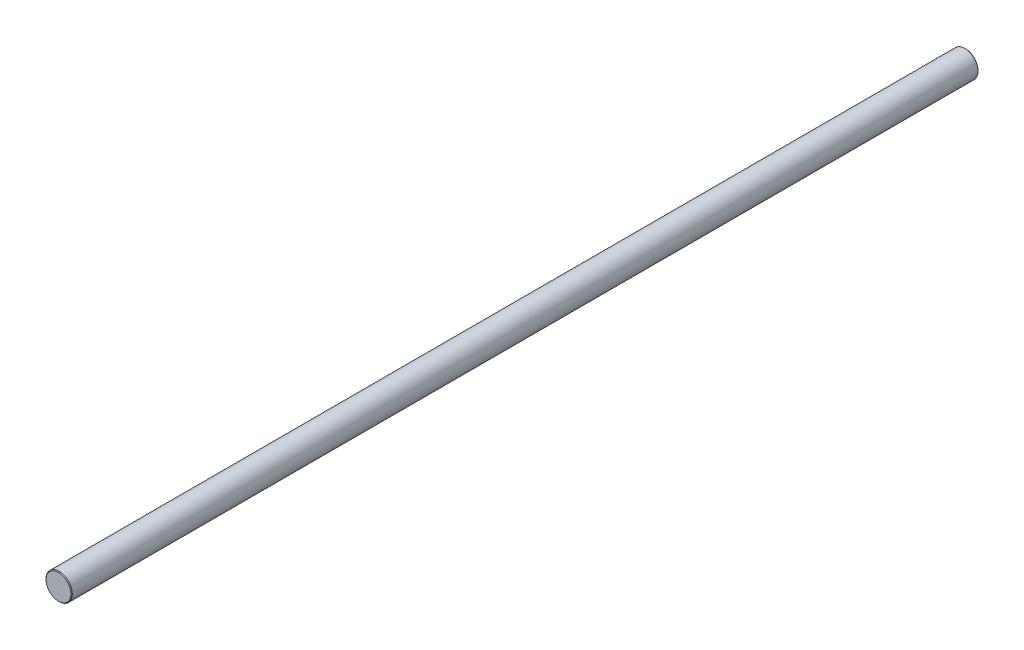
from build123d import *

# Parameters (mm, degrees)
SKETCH_1_R      = 10
EXTRUDE_1_DEPTH = 345
CHAMFER_1_SIZE  = 0.5


with BuildPart() as part:
    # 草图1 → 凸台-拉伸1 (new, symmetric)
    with BuildSketch(Plane.XY):
        with Locations(Location((0, 0, 0), (0, 0, 180))):
            Circle(SKETCH_1_R)
    extrude(amount=EXTRUDE_1_DEPTH, both=True)

    # 倒角1
    chamfer_1_edges = [part.edges().sort_by_distance(p)[0] for p in [
        (10, 0, -345),
        (10, 0, 345),
    ]]
    chamfer(chamfer_1_edges, length=CHAMFER_1_SIZE)


solid = part.part
